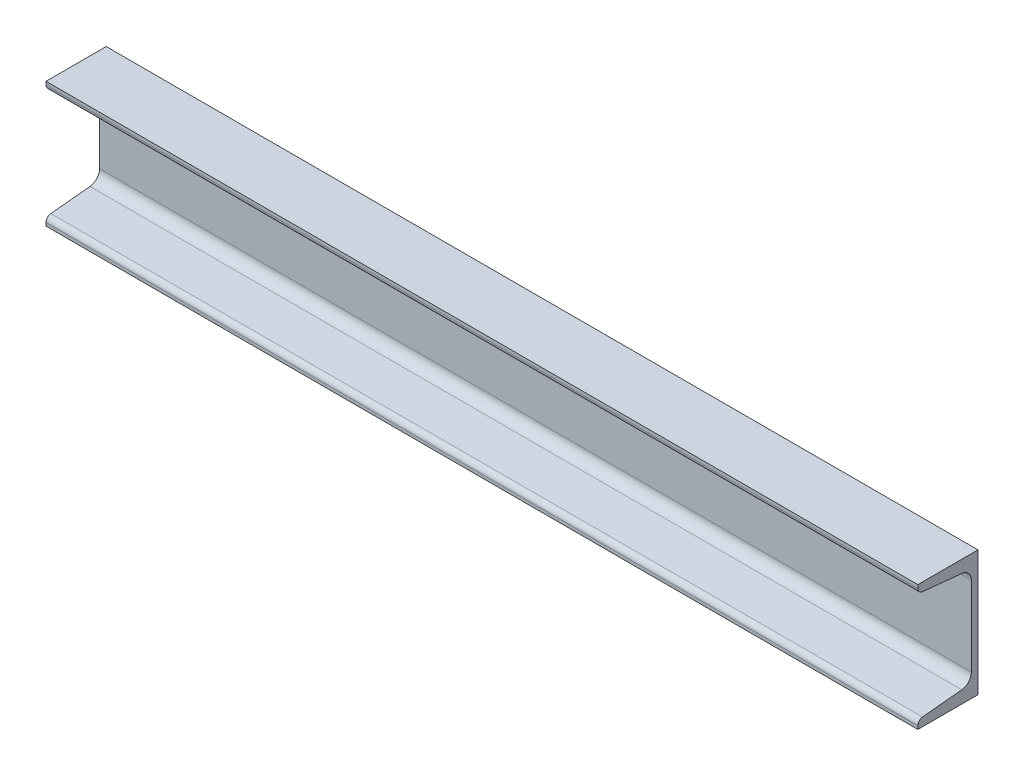
from build123d import *

# Parameters (mm, degrees)
BASE_DEPTH = 695
FILLET1_R  = 8.5
FILLET2_R  = 4.25


with BuildPart() as part:
    # Sketch1 → Base (new body)
    with BuildSketch(Plane(origin=(0, 0, -28.211262136), x_dir=(0, 0, 1), z_dir=(1, 0, 0))):
        Polygon((28.211262136, -50), (28.211262136, 50), (76.211262136, 50), (76.211262136, 43.635), (33.511262136, 39.365), (33.511262136, -39.365), (76.211262136, -43.635), (76.211262136, -50), align=None)
    extrude(amount=BASE_DEPTH)

    # Fillet1
    fillet1_edges = [part.edges().sort_by_distance(p)[0] for p in [
        (347.5, -39.365, 5.3),
        (347.5, 39.365, 5.3),
    ]]
    fillet(fillet1_edges, radius=FILLET1_R)

    # Fillet2
    fillet2_edges = [part.edges().sort_by_distance(p)[0] for p in [
        (347.5, 43.635, 48),
        (347.5, -43.635, 48),
    ]]
    fillet(fillet2_edges, radius=FILLET2_R)


solid = part.part
